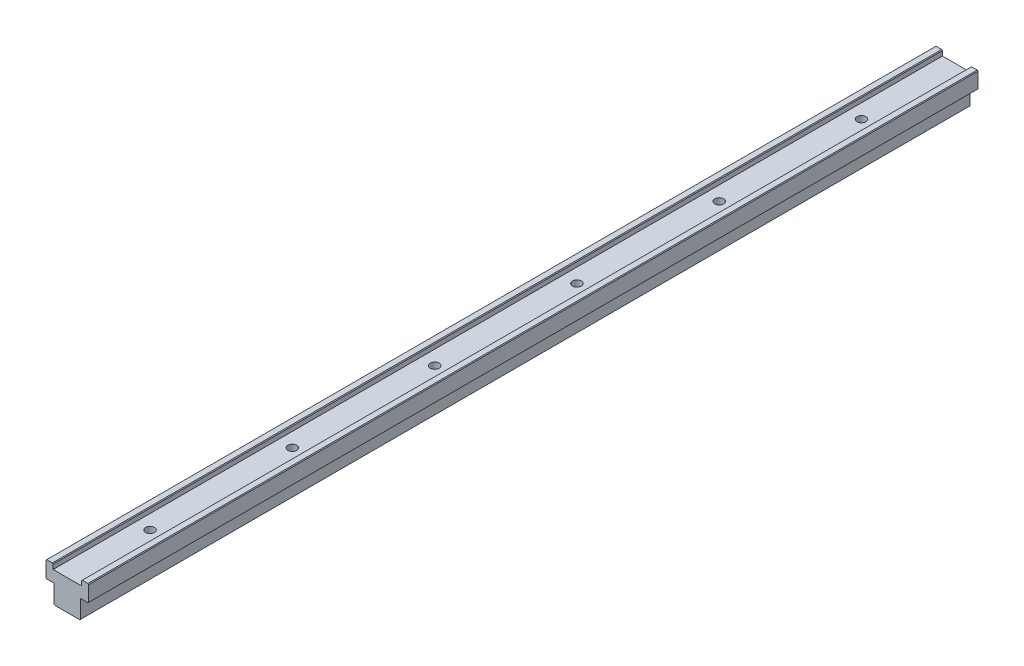
SolidWorks part; units mm, degrees
ref_plane "Front Plane" through (0, 0, 0) normal (0, 0, 1) x (1, 0, 0)
ref_plane "Top Plane" through (0, 0, 0) normal (0, 1, 0) x (1, 0, 0)
ref_plane "Right Plane" through (0, 0, 0) normal (1, 0, 0) x (0, 0, -1)
sketch "Sketch1" plane through (0, 0, 0) normal (0, 0, 1) x (1, 0, 0)
  line L0 (0, 4.8581) -> (0, -11.7093) construction
  line L5 (4, 0) -> (-4, 0)
  line L6 (-4, 0) -> (-4, 1.5)
  line L7 (-4, 1.5) -> (-6, 1.5)
  line L8 (-6, 1.5) -> (-6, -3.2)
  line L9 (-6, -3.2) -> (-3.7, -3.2)
  line L10 (-3.7, -3.2) -> (-3.7, -8.5)
  line L11 (-3.7, -8.5) -> (3.7, -8.5)
  line L12 (3.7, -3.2) -> (3.7, -8.5)
  line L13 (6, -3.2) -> (3.7, -3.2)
  line L14 (6, 1.5) -> (6, -3.2)
  line L15 (4, 1.5) -> (6, 1.5)
  line L16 (4, 0) -> (4, 1.5)
  point P15 (0, -8.5)
  point P20 (0, 0)
  dimension "D1" = 12
  dimension "D2" = 2
  dimension "D3" = 1.5
  dimension "D4" = 5.3
  dimension "D5" = 2.3
  dimension "D6" = 10
extrude "Boss-Extrude1" add sketch "Sketch1" along normal mid plane 250
hole_wizard "M3 Tapped Hole1" positions "Sketch2" profile "Sketch3" tap size "M3" standard "GB" end condition through all
sketch "Sketch2" plane through (0, 0, 0) normal (0, 1, 0) x (1, 0, 0)
  point P0 (0, 98.25)
sketch "Sketch3" plane through (0, 0, -98.25) normal (1, 0, 0) x (0, 0, 1)
  line L0 (0, 0) -> (0, 8.5)
  line L1 (0, 8.5) -> (1.25, 8.5)
  line L2 (1.25, 8.5) -> (1.25, 0)
  line L5 (1.25, 0) -> (0, 0)
  line L11 (0, -6.35) -> (0, 107.95) construction
  dimension "通孔螺纹孔钻头直径" = 2.5
  dimension "通孔螺纹孔钻头深度" = 8.5
cosmetic thread "Cosmetic Thread1" parameters "D2"=3
chamfer "Chamfer1" distance 0.2 angle 45 8 edges at (-6, 1.5, 0) (-6, -3.2, 0) (-3.7, -8.5, 0) (3.7, -8.5, 0) (6, -3.2, 0) (6, 1.5, 0) (-4, 1.5, 0) (4, 1.5, 0)
pattern_linear "LPattern1" count 6 spacing 40 along (0, 0, 1) of "M3 Tapped Hole1"
cosmetic thread "Cosmetic Thread2" parameters "D2"=3
cosmetic thread "Cosmetic Thread3" parameters "D2"=3
cosmetic thread "Cosmetic Thread4" parameters "D2"=3
cosmetic thread "Cosmetic Thread5" parameters "D2"=3
cosmetic thread "Cosmetic Thread6" parameters "D2"=3
equation "\"1\"= \"代号代号\""
equation "\"2\"= \"名称代号\""
